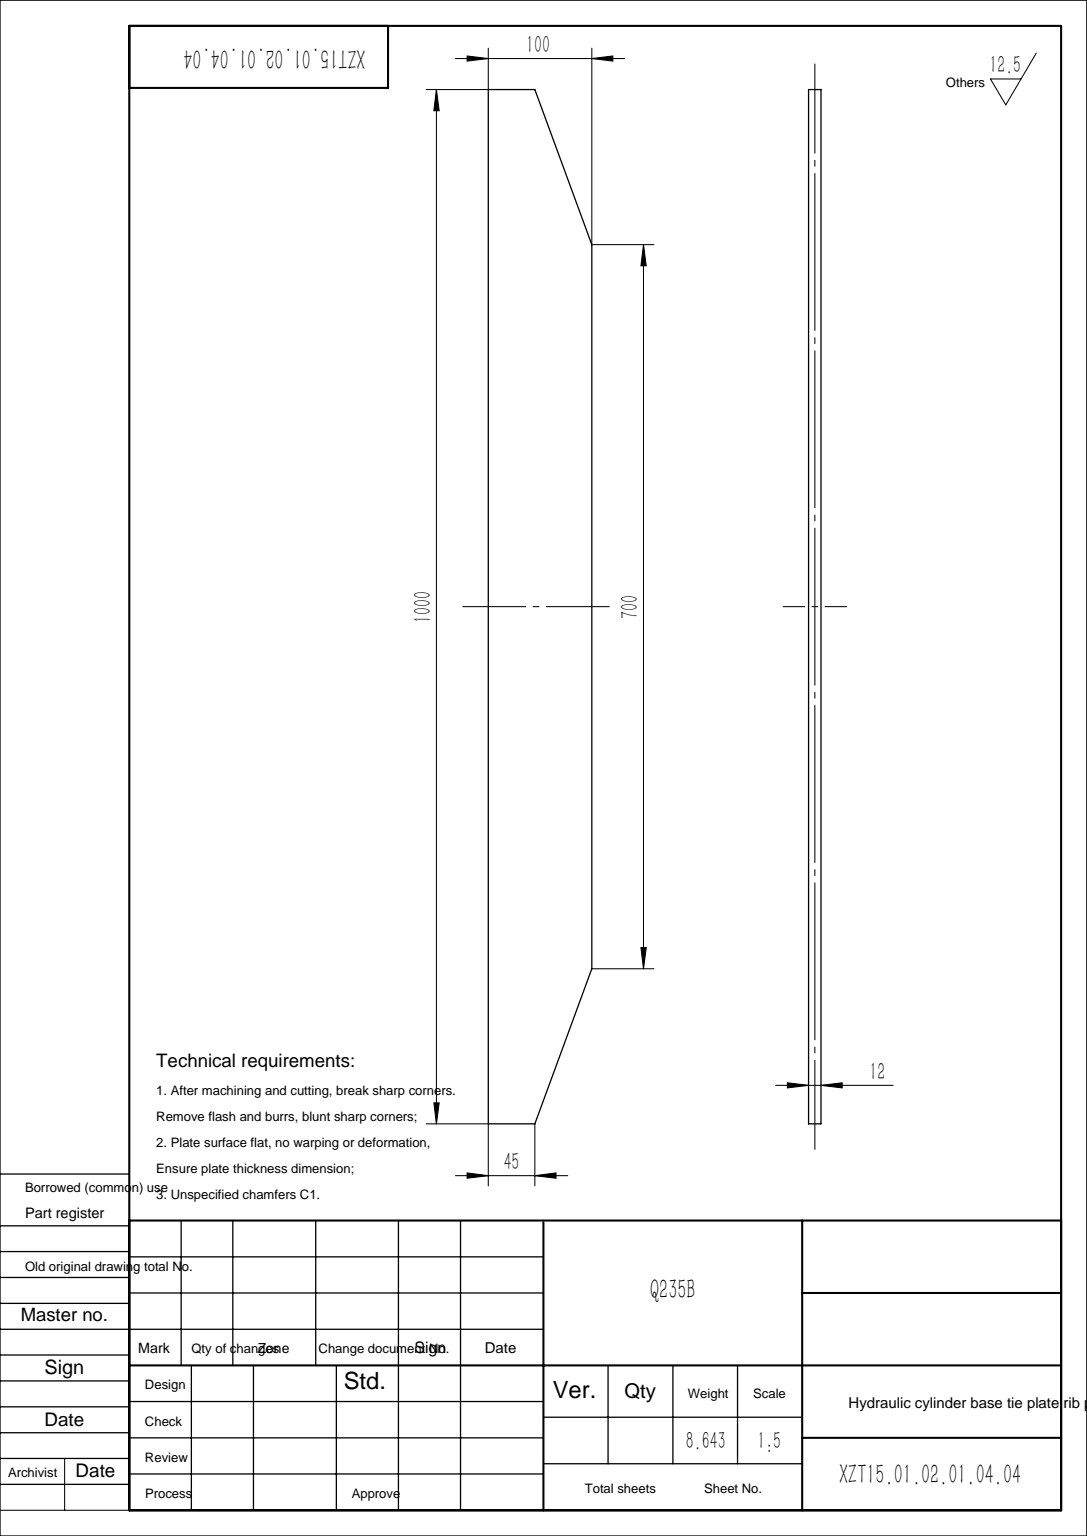
from build123d import *

# Parameters (mm, degrees)
BOSS_EXTRUDE1_DEPTH = 6


with BuildPart() as part:
    # Sketch1 → Boss-Extrude1 (new, symmetric)
    with BuildSketch(Plane.XY):
        Polygon((0, -500), (0, 500), (45, 500), (100, 350), (100, -350), (45, -500), align=None)
    extrude(amount=BOSS_EXTRUDE1_DEPTH, both=True)


solid = part.part
